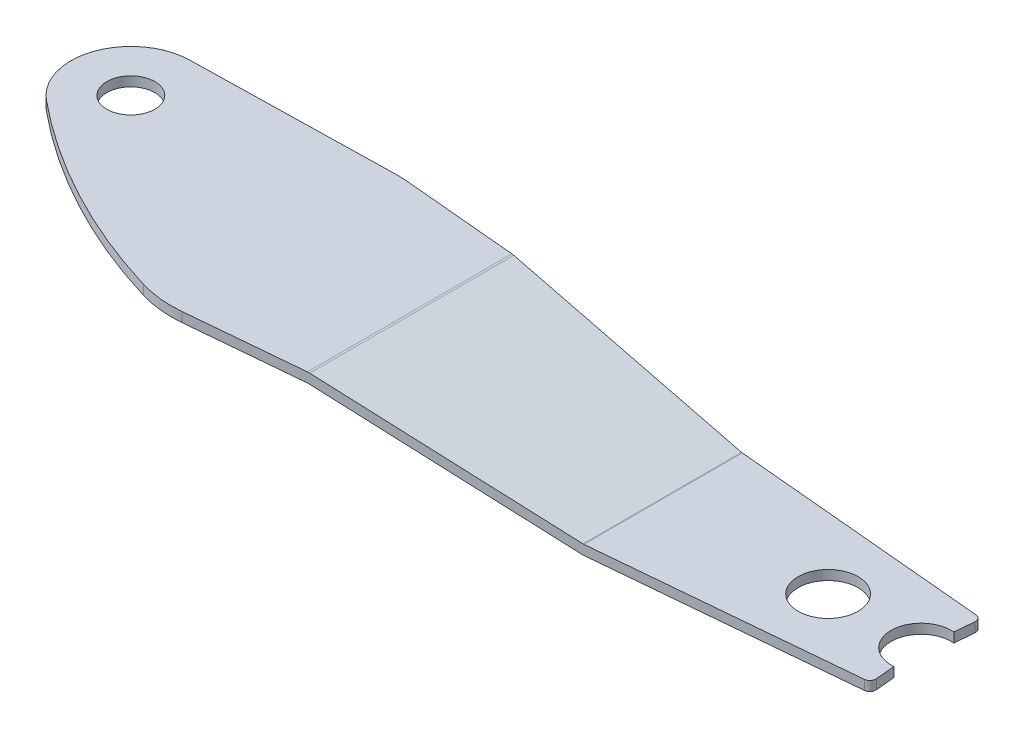
SolidWorks part; units mm, degrees
ref_plane "Front Plane" through (0, 0, 0) normal (0, 0, 1) x (1, 0, 0)
ref_plane "Top Plane" through (0, 0, 0) normal (0, 1, 0) x (1, 0, 0)
ref_plane "Right Plane" through (0, 0, 0) normal (1, 0, 0) x (0, 0, -1)
sketch "Sketch1" plane through (0, 0, 0) normal (0, 0, 1) x (1, 0, 0)
  line L0 (0, 0) -> (-547.3, 0) construction
  line L1 (419.8, -57) -> (851, -57) construction
  line L2 (0, 0) -> (419.8, -57) construction
  line L3 (-1.2164, 8) -> (-647.3, 8)
  line L4 (2.2817, 7.7636) -> (419.671, -48.9091)
  line L5 (421.0164, -49) -> (943.5, -49)
  line L6 (-647.3, 8) -> (-647.3, -8)
  line L7 (0, 8) -> (-547.3, 8) construction
  line L8 (943.5, -49) -> (943.5, -65)
  line L9 (419.8, -49) -> (851, -49) construction
  line L10 (421.0164, -65) -> (943.5, -65)
  line L11 (0.129, -8.0909) -> (417.5183, -64.7636)
  line L12 (-1.2164, -8) -> (-647.3, -8)
  line L13 (0, -8) -> (-647.3, -8) construction
  line L14 (-1.0764, -7.9273) -> (418.7236, -64.9273) construction
  line L15 (1.0764, 7.9273) -> (420.8764, -49.0727) construction
  line L16 (419.8, -49) -> (943.5, -49) construction
  line L17 (0, 8) -> (-647.3, 8) construction
  line L18 (419.8, -65) -> (943.5, -65) construction
  arc A0 (-1.2164, -8) -> (0.129, -8.0909) centre (-1.2164, -18) cw
  arc A1 (419.671, -48.9091) -> (421.0164, -49) centre (421.0164, -39) ccw
  arc A2 (2.2817, 7.7636) -> (-1.2164, 8) centre (-1.2164, -18) ccw
  arc A3 (421.0164, -65) -> (417.5183, -64.7636) centre (421.0164, -39) cw
  dimension "D13" = 10
  dimension "D14" = 10
  dimension "D15" = 26
  dimension "D16" = 26
  dimension "D1" = 547.3
  dimension "D2" = 57
  dimension "D3" = 1398.3
  dimension "D4" = 431.2
  dimension "D8" = 100
  dimension "D9" = 92.5
  dimension "D5" = 8
  dimension "D6" = 8
  dimension "D7" = 8
  dimension "D10" = 16
  dimension "D11" = 16
  dimension "D12" = 16
extrude "Boss-Extrude1" add sketch "Sketch1" along normal blind 600
sketch "Sketch4" plane through (0, 8, 0) normal (0, 1, 0) x (1, 0, 0)
  line L0 (0, 0) -> (0, -1359.8817) construction
  line L1 (-547.3, -1279.6671) -> (-547.3, 561.2691) construction
  line L2 (-647.3, -600) -> (-647.3, 0) construction
  line L3 (-647.3, -300) -> (1324.1271, -300) construction
  line L4 (-647.3, -600) -> (-647.3, 0) construction
  line L5 (-616.4551, -218.5) -> (-263.7468, -218.5) construction
  line L6 (-209.8, -1329.3592) -> (-209.8, 330.295) construction
  line L7 (849.441, -393.0228) -> (-192.7412, -487.7265)
  line L8 (849.441, -206.9772) -> (-192.7412, -112.2735)
  line L9 (-549.3793, -118.5216) -> (-213.7195, -111.5408)
  line L10 (858.495, -382.1588) -> (855.5538, -349.7922)
  line L11 (851, -1009.9733) -> (851, 231.9619) construction
  line L12 (696, -822.7119) -> (696, 170.4845) construction
  line L13 (858.495, -217.8412) -> (855.5538, -250.2078)
  circle A0 centre (-547.3, -218.5) radius 40
  arc A1 (-549.3793, -118.5216) -> (-610.7425, -295.7985) centre (-547.3, -218.5) ccw
  arc A2 (-264.0347, -480.5294) -> (-192.7412, -487.7265) centre (-209.8, -300) ccw
  arc A3 (859.371, -392.1204) -> (859.371, -207.8796) centre (851, -300) ccw construction
  arc A4 (855.5538, -250.2078) -> (855.5538, -349.7922) centre (851, -300) ccw
  circle A5 centre (696, -300) radius 50
  arc A6 (-610.7425, -295.7985) -> (-264.0347, -480.5294) centre (23.6823, 477.1861) ccw
  arc A7 (-192.7412, -112.2735) -> (-213.7195, -111.5408) centre (-209.8, -300) ccw
  arc A8 (849.441, -206.9772) -> (858.495, -217.8412) centre (848.5361, -216.9362) cw
  arc A9 (849.441, -393.0228) -> (858.495, -382.1588) centre (848.5361, -383.0638) ccw
  point P39 (859.4, -207.8822)
  point P43 (859.4, -392.1178)
  dimension "D3" = 80
  dimension "D4" = 200
  dimension "D7" = 2000
  dimension "D10" = 185
  dimension "D11" = 100
  dimension "D12" = 100
  dimension "D6" = 377
  dimension "D8" = 8.4
  dimension "D14" = 10
  dimension "D1" = 100
  dimension "D2" = 81.5
  dimension "D5" = 337.5
  dimension "D9" = 1398.3
  dimension "D13" = 155
extrude "Cut-Extrude1" cut sketch "Sketch4" against normal through all flip side to cut
